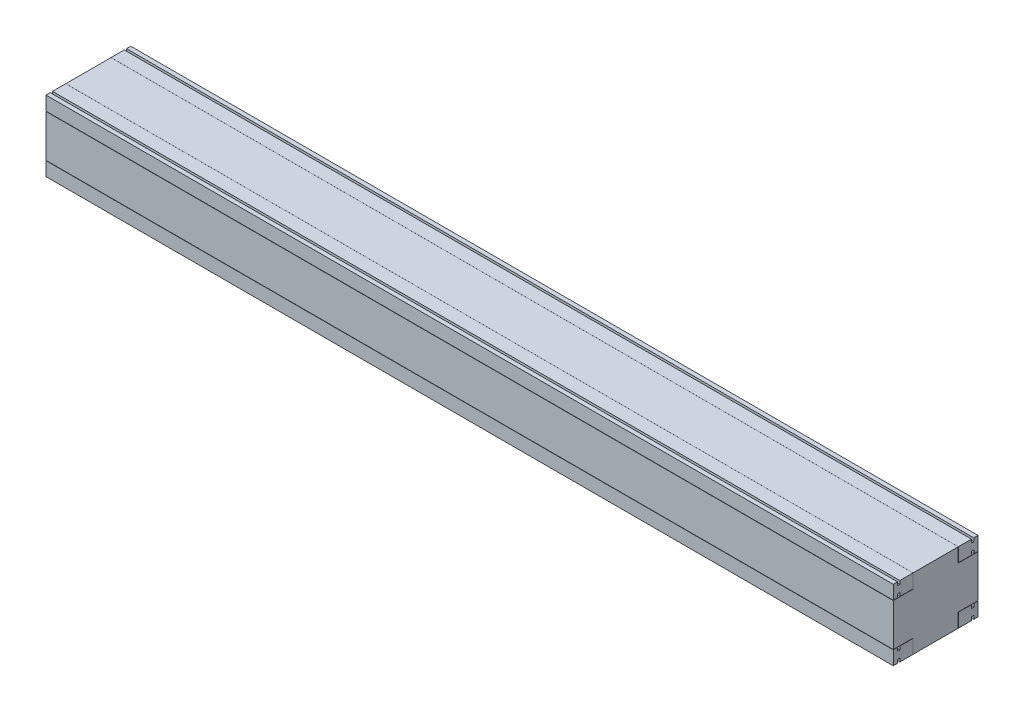
SolidWorks part; units mm, degrees
ref_plane "Front Plane" through (0, 0, 0) normal (0, 0, 1) x (1, 0, 0)
ref_plane "Top Plane" through (0, 0, 0) normal (0, 1, 0) x (1, 0, 0)
ref_plane "Right Plane" through (0, 0, 0) normal (1, 0, 0) x (0, 0, -1)
other "Configuration Table"
sketch "Sketch1" plane through (0, 0, 0) normal (0, 1, 0) x (1, 0, 0)
  line L1 (-1500, 150) -> (1500, 150)
  line L2 (-1500, 150) -> (-1500, -150)
  line L3 (-1500, -150) -> (1500, -150)
  line L4 (1500, 150) -> (1500, -150)
  line L5 (-1500, 150) -> (1500, -150) construction
  line L6 (-1500, -150) -> (1500, 150) construction
  point P0 (0, 0)
  dimension "D1" = 300
  dimension "D2" = 3000
extrude "Boss-Extrude1" add sketch "Sketch1" along normal blind 250
sketch "Sketch2" plane through (1500, 0, 0) normal (1, 0, 0) x (0, 0, -1)
  line L0 (-150, 250) -> (150, 0) construction
  line L1 (150, 250) -> (150, 0) construction
  line L2 (-150, 200) -> (-80, 200)
  line L4 (-150, 50) -> (-80, 50)
  line L6 (-150, 200) -> (150, 50) construction
  line L7 (-150, 50) -> (150, 200) construction
  line L8 (-150, 0) -> (150, 0) construction
  line L10 (-80, 250) -> (-80, 200)
  line L12 (80, 250) -> (80, 200)
  line L13 (-80, 250) -> (80, 0) construction
  line L14 (-80, 0) -> (80, 250) construction
  line L15 (-150, 250) -> (-150, 0) construction
  line L16 (80, 200) -> (150, 200)
  line L17 (-150, 200) -> (-150, 250)
  line L18 (80, 50) -> (80, 0)
  line L19 (80, 50) -> (150, 50)
  line L20 (-80, 50) -> (-80, 0)
  line L21 (-150, 250) -> (-80, 250)
  line L22 (80, 250) -> (150, 250)
  line L23 (150, 250) -> (150, 200)
  line L24 (150, 50) -> (150, 0)
  line L25 (150, 0) -> (80, 0)
  line L26 (-80, 0) -> (-150, 0)
  line L27 (-150, 0) -> (-150, 50)
  point P4 (0, 125)
  point P11 (0, 125)
  dimension "D1" = 50
  dimension "D2" = 70
extrude "Cut-Extrude1" cut sketch "Sketch2" against normal through all
sketch "Sketch3" plane through (1500, 0, 0) normal (1, 0, 0) x (0, 0, -1)
  line L0 (135, 250) -> (135, 238)
  line L1 (80.2, 250) -> (127, 250)
  line L2 (80.2, 250) -> (80.2, 201)
  line L3 (80.2, 201) -> (127, 201)
  line L4 (150, 250) -> (150, 201)
  line L5 (135, 238) -> (127, 238)
  line L6 (127, 238) -> (127, 250)
  line L7 (135, 201) -> (135, 213)
  line L8 (135, 213) -> (127, 213)
  line L9 (127, 213) -> (127, 201)
  line L10 (135, 250) -> (150, 250)
  line L12 (135, 201) -> (150, 201)
  line L13 (80, 200) -> (150, 200) construction
  line L14 (150, 200) -> (150, 50) construction
  line L15 (80, 250) -> (80, 200) construction
  dimension "D1" = 8
  dimension "D2" = 12
  dimension "D3" = 8
  dimension "D4" = 12
  dimension "D5" = 15
  dimension "D6" = 1
  dimension "D7" = 0.2
extrude "Boss-Extrude2" add sketch "Sketch3" against normal up to surface (3000 mm away) up to face at (-1500, 125, 0)
ref_plane "Plane2" through (0, 125, 0) normal (0, -1, 0) x (-1, 0, 0)
mirror "Mirror3" about plane through (0, 125, 0) normal (0, -1, 0) of bodies 108
mirror "Mirror4" about plane through (0, 0, 0) normal (0, 0, 1) of bodies 109 108
